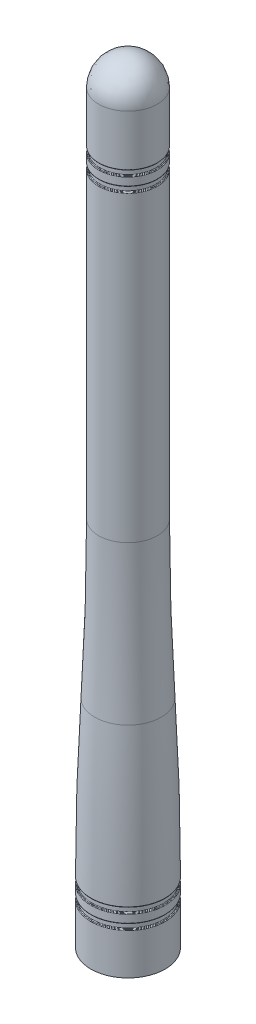
from build123d import *

# Parameters (mm, degrees)
FILLET1_R = 0.08


with BuildPart() as part:
    # Sketch2 → Revolve1 (revolve)
    with BuildSketch(Plane.XY, mode=Mode.PRIVATE) as revolve1_sk:
        with BuildLine():
            Line((-5, 0), (-5, 5.609800729))
            Line((-5, 5.609800729), (-4.8, 5.609800729))
            Line((-4.8, 5.609800729), (-4.8, 6.309800729))
            Line((-4.8, 6.309800729), (-5, 6.309800729))
            Line((-5, 6.309800729), (-5, 7.509800729))
            Line((-5, 7.509800729), (-4.8, 7.509800729))
            Line((-4.8, 7.509800729), (-4.8, 8.209800729))
            Line((-4.8, 8.209800729), (-5, 8.209800729))
            ThreePointArc((-5, 8.209800729), (-4.868729867, 18.660601983), (-4.475002299, 29.104808861))
            ThreePointArc((-4.475002299, 29.104808861), (-4.081271283, 39.549107214), (-3.95, 50))
            Line((-3.95, 50), (-3.95, 90.8))
            Line((-3.95, 90.8), (-3.75, 90.8))
            Line((-3.75, 90.8), (-3.75, 91.5))
            Line((-3.75, 91.5), (-3.95, 91.5))
            Line((-3.95, 91.5), (-3.95, 92.7))
            Line((-3.95, 92.7), (-3.75, 92.7))
            Line((-3.75, 92.7), (-3.75, 93.4))
            Line((-3.75, 93.4), (-3.95, 93.4))
            Line((-3.95, 93.4), (-3.95, 100.3))
            ThreePointArc((-3.95, 100.3), (-2.789981752, 103.075337817), (0, 104.199679474))
            Line((0, 104.199679474), (0, 100.3))
            Line((0, 100.3), (-2.95211686, 100.3))
            Line((-2.95211686, 100.3), (-2.95211686, 50))
            ThreePointArc((-2.95211686, 50), (-3.149910758, 37.156662475), (-3.74310485, 24.325506566))
            ThreePointArc((-3.74310485, 24.325506566), (-3.785772839, 23.402571518), (-3.8, 22.478760255))
            Line((-3.8, 22.478760255), (-3.8, 4))
            Line((-3.8, 4), (-4, 4))
            Line((-4, 4), (-4, 3.5))
            Line((-4, 3.5), (-3.8, 3.5))
            Line((-3.8, 3.5), (-3.8, 3))
            Line((-3.8, 3), (-4, 3))
            Line((-4, 3), (-4, 2.5))
            Line((-4, 2.5), (-3.8, 2.5))
            Line((-3.8, 2.5), (-3.8, 2))
            Line((-3.8, 2), (-4, 2))
            Line((-4, 2), (-4, 1.5))
            Line((-4, 1.5), (-3.8, 1.5))
            Line((-3.8, 1.5), (-3.8, 0))
            Line((-3.8, 0), (-5, 0))
        make_face()
    revolve(revolve1_sk.sketch.rotate(Axis((0, 110.08841758, 0), (0, -1, 0)), 270), axis=Axis((0, 110.08841758, 0), (0, -1, 0)))

    # Fillet1
    fillet1_edges = [part.edges().sort_by_distance(p)[0] for p in [
        (0, 5.609800729, -5),
        (0, 5.609800729, -4.8),
        (0, 6.309800729, -4.8),
        (0, 6.309800729, -5),
        (0, 7.509800729, -5),
        (0, 7.509800729, -4.8),
        (0, 8.209800729, -4.8),
        (0, 8.209800729, -5),
        (0, 90.8, -3.95),
        (0, 90.8, -3.75),
        (0, 91.5, -3.75),
        (0, 91.5, -3.95),
        (0, 92.7, -3.95),
        (0, 92.7, -3.75),
        (0, 93.4, -3.75),
        (0, 93.4, -3.95),
    ]]
    fillet(fillet1_edges, radius=FILLET1_R)


solid = part.part
